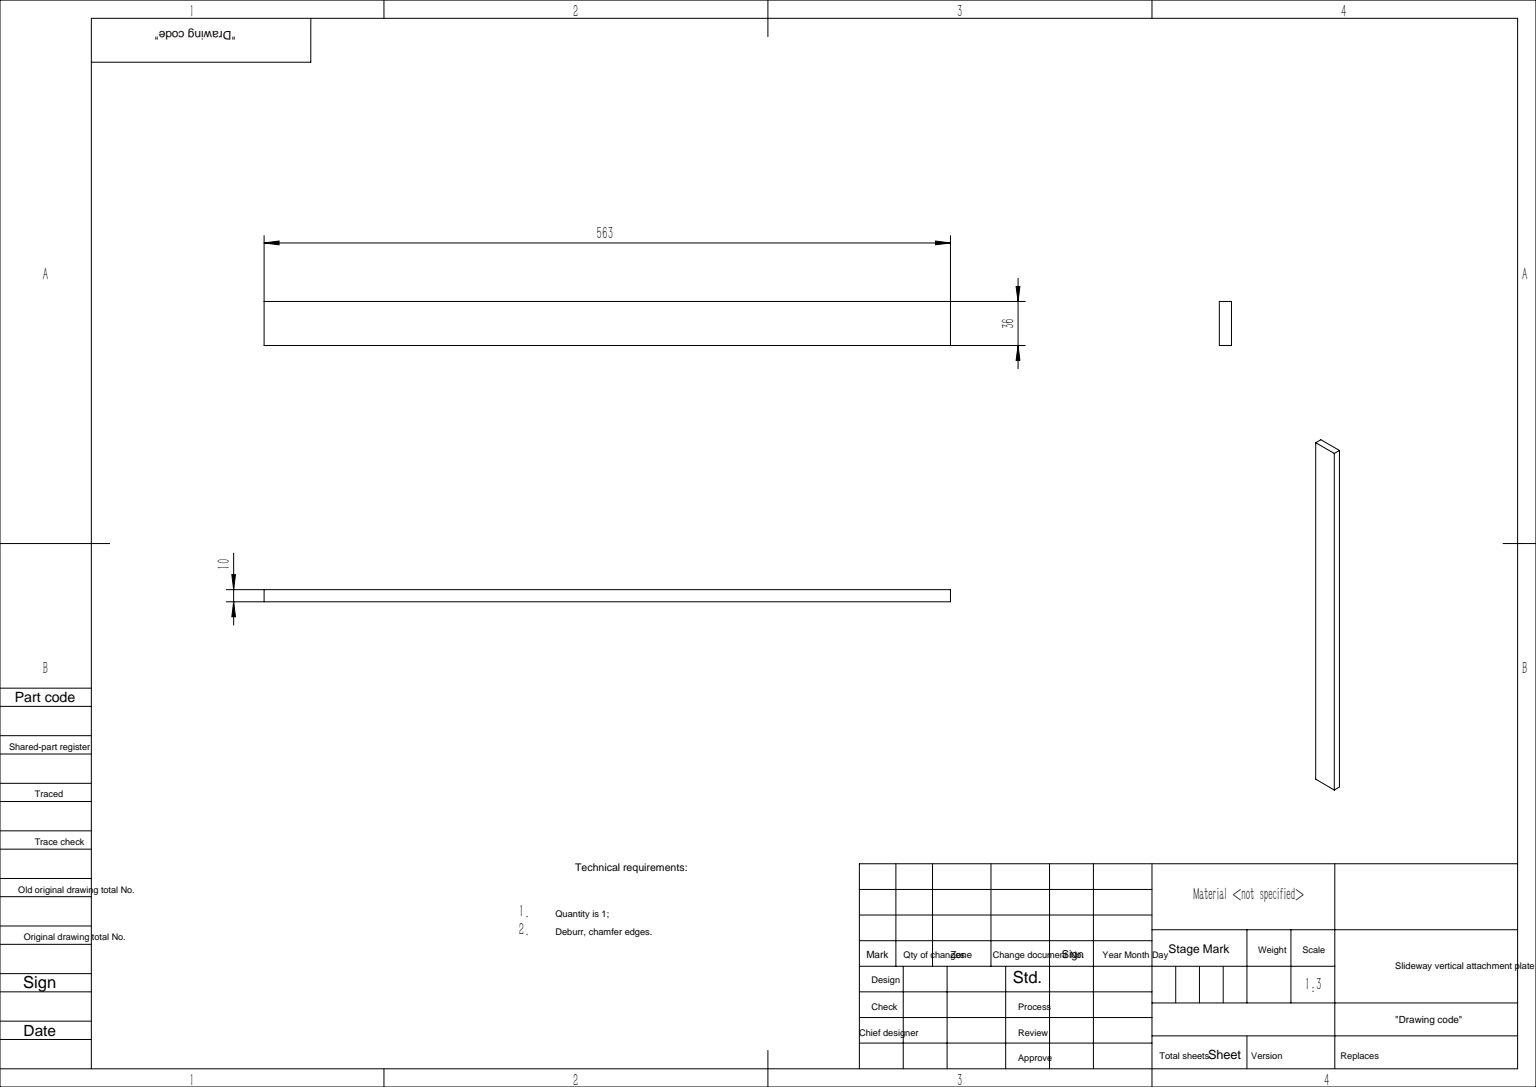
SolidWorks part; units mm, degrees
ref_plane "前视基准面" through (0, 0, 0) normal (0, 0, 1) x (1, 0, 0)
ref_plane "上视基准面" through (0, 0, 0) normal (0, 1, 0) x (1, 0, 0)
ref_plane "右视基准面" through (0, 0, 0) normal (1, 0, 0) x (0, 0, -1)
sketch "草图1" plane through (0, 30, 0) normal (0, 1, 0) x (1, 0, 0)
  line L0 (18, 6) -> (18, 10) construction
  line L1 (-18, 10) -> (18, 10)
  line L2 (-18, 10) -> (-18, 20)
  line L3 (-18, 20) -> (18, 20)
  line L4 (18, 10) -> (18, 20)
  dimension "D1" = 10
extrude "凸台-拉伸1" add sketch "草图1" along normal up to vertex (563 mm away)
